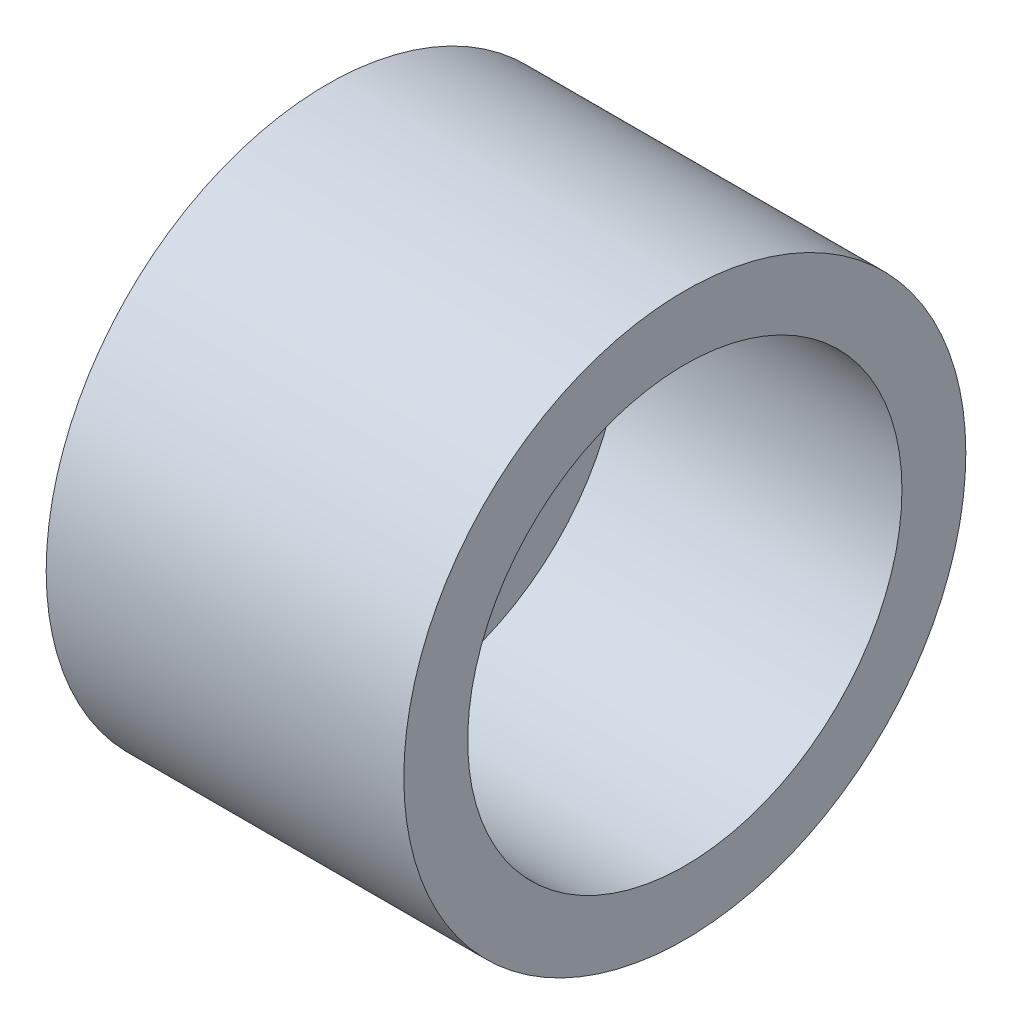
from build123d import *

# Parameters (mm, degrees)
SKETCH1_R           = 5.5
SKETCH1_R_2         = 2.75
BOSS_EXTRUDE1_DEPTH = 7
SKETCH2_R           = 4.25
CUT_EXTRUDE1_DEPTH  = 5.5


with BuildPart() as part:
    # Sketch1 → Boss-Extrude1 (new body)
    with BuildSketch(Plane(origin=(0, 0, 0), x_dir=(0, 0, -1), z_dir=(1, 0, 0))):
        Circle(SKETCH1_R)
        Circle(SKETCH1_R_2, mode=Mode.SUBTRACT)
    extrude(amount=BOSS_EXTRUDE1_DEPTH)

    # Sketch2 → Cut-Extrude1 (cut)
    with BuildSketch(Plane(origin=(7, 0, 0), x_dir=(0, 0, -1), z_dir=(1, 0, 0))):
        Circle(SKETCH2_R)
    extrude(amount=-CUT_EXTRUDE1_DEPTH, mode=Mode.SUBTRACT)


solid = part.part
